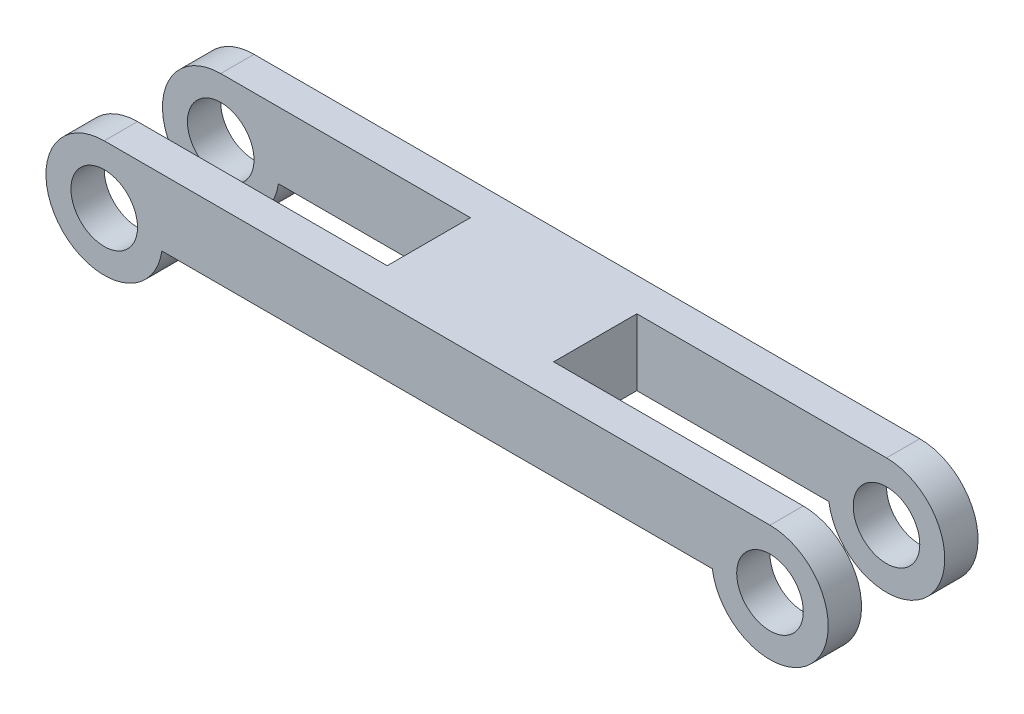
from build123d import *

# Parameters (mm, degrees)
SKETCH1_R           = 2
BOSS_EXTRUDE1_DEPTH = 9
SKETCH2_W           = 37
SKETCH2_H           = 5
CUT_EXTRUDE1_DEPTH  = 9


with BuildPart() as part:
    # Sketch1 → Boss-Extrude1 (new body)
    with BuildSketch(Plane.XY):
        with BuildLine():
            Line((-20, 3.5), (20, 3.5))
            ThreePointArc((20, 3.5), (22.645751311, -2.291287847), (16.535898385, -0.5))
            Line((16.535898385, -0.5), (-16.535898385, -0.5))
            ThreePointArc((-16.535898385, -0.5), (-22.645751311, -2.291287847), (-20, 3.5))
        make_face()
        with Locations((20, 0)):
            Circle(SKETCH1_R, mode=Mode.SUBTRACT)
        with Locations((-20, 0)):
            Circle(SKETCH1_R, mode=Mode.SUBTRACT)
    extrude(amount=BOSS_EXTRUDE1_DEPTH)

    # Sketch2 → Cut-Extrude1 (cut)
    with BuildSketch(Plane(origin=(0, 3.5, 0), x_dir=(1, 0, 0), z_dir=(0, 1, 0))):
        with Locations((-23.5, -4.5)):
            Rectangle(SKETCH2_W, SKETCH2_H)
    cut_extrude1 = extrude(amount=-CUT_EXTRUDE1_DEPTH, mode=Mode.SUBTRACT)

    # Mirror1: Cut-Extrude1 across plane
    add(cut_extrude1.mirror(Plane(origin=(0, 0, 0), x_dir=(0, 0, 1), z_dir=(1, 0, 0))), mode=Mode.SUBTRACT)


solid = part.part
